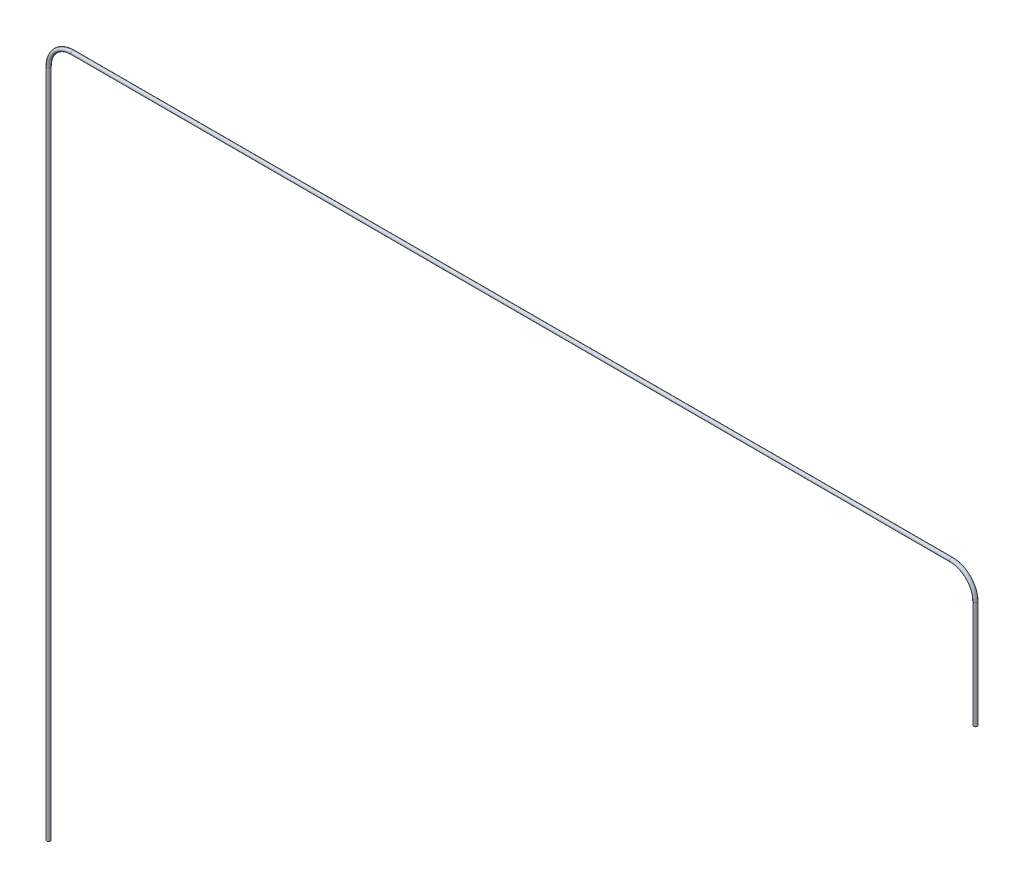
SolidWorks part; units mm, degrees
ref_plane "Front Plane" through (0, 0, 0) normal (0, 0, 1) x (1, 0, 0)
ref_plane "Top Plane" through (0, 0, 0) normal (0, 1, 0) x (1, 0, 0)
ref_plane "Right Plane" through (0, 0, 0) normal (1, 0, 0) x (0, 0, -1)
sketch "Sketch1" plane through (0, 0, 0) normal (0, 0, 1) x (1, 0, 0)
  line L0 (0, 0) -> (0, 1173)
  line L1 (42, 1215) -> (1580, 1215)
  line L2 (1622, 1173) -> (1622, 985)
  arc A0 (1580, 1215) -> (1622, 1173) centre (1580, 1173) cw
  arc A1 (0, 1173) -> (42, 1215) centre (42, 1173) cw
  point P7 (1622, 1215)
  point P10 (0, 1215)
  dimension "D3" = 42
  dimension "D1" = 1622
  dimension "D2" = 1215
  dimension "D4" = 230
sketch "Sketch2" plane through (0, 0, 0) normal (0, 1, 0) x (1, 0, 0)
  circle A0 centre (0, 0) radius 3.25
  dimension "D1" = 6.5
sweep "Sweep1" add profiles "Sketch2" path "Sketch1"
